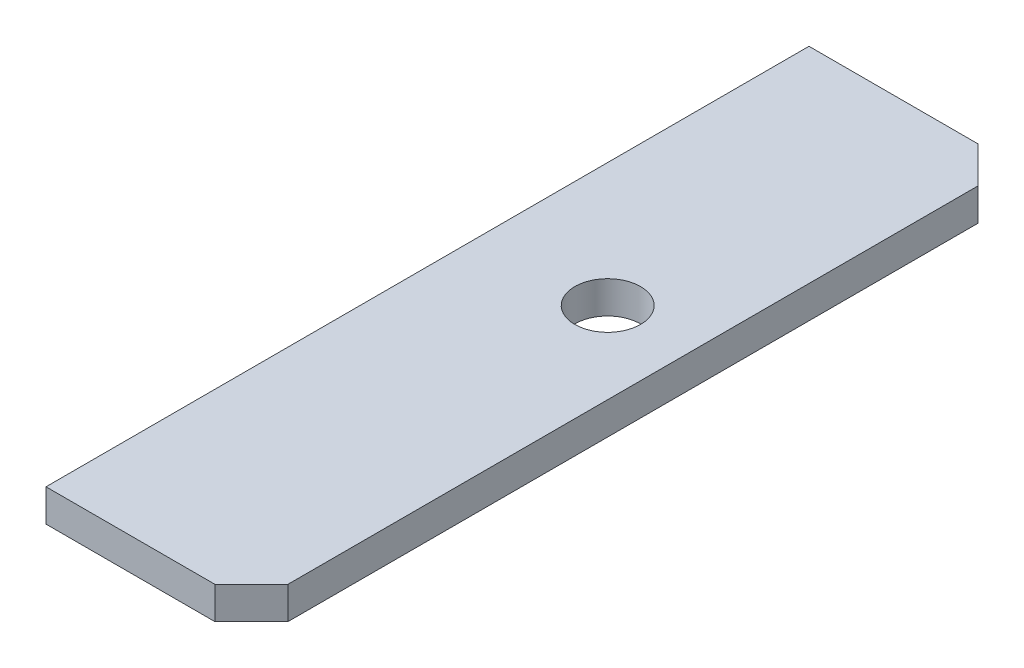
SolidWorks part; units mm, degrees
material "普通碳钢"
ref_plane "Front Plane" through (0, 0, 0) normal (0, 0, 1) x (1, 0, 0)
ref_plane "Top Plane" through (0, 0, 0) normal (0, 1, 0) x (1, 0, 0)
ref_plane "Right Plane" through (0, 0, 0) normal (1, 0, 0) x (0, 0, -1)
sketch "Sketch3" plane through (0, 0, 0) normal (0, 1, 0) x (1, 0, 0)
  line L0 (19.556, 140.716) -> (35.306, 124.966)
  line L1 (-53.594, 140.716) -> (19.556, 140.716)
  line L2 (-53.594, 140.716) -> (-53.594, -189.484)
  line L3 (-53.594, -189.484) -> (19.556, -189.484)
  line L4 (35.306, 124.966) -> (35.306, -173.734)
  line L5 (35.306, -173.734) -> (19.556, -189.484)
  circle A0 centre (0, 0) radius 14.224
  point P1 (35.306, -189.484)
  point P3 (35.306, 140.716)
  dimension "D3" = 35.306
  dimension "D7" = 28.448
  dimension "D1" = 88.9
  dimension "D2" = 330.2
  dimension "D4" = 140.716
extrude "Boss-Extrude1" add sketch "Sketch3" along normal mid plane 14
